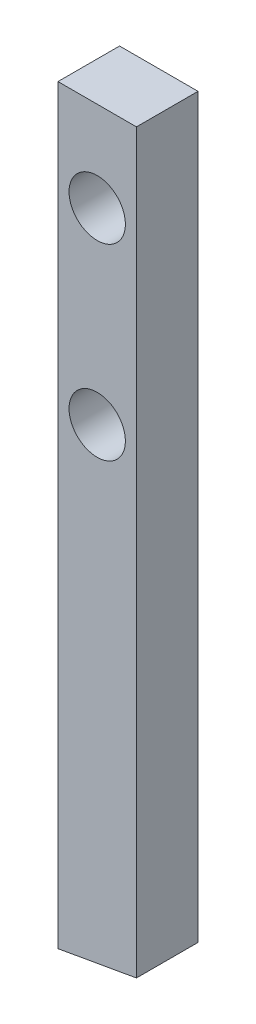
from build123d import *

# Parameters (mm, degrees)
SKETCH1_W           = 4.18
SKETCH1_H           = 3.28
BOSS_EXTRUDE1_DEPTH = 40
CUT_EXTRUDE1_DEPTH  = 40
SKETCH3_R           = 1.5
CUT_EXTRUDE2_DEPTH  = 40


with BuildPart() as part:
    # Sketch1 → Boss-Extrude1 (new body)
    with BuildSketch(Plane(origin=(0, 0, 0), x_dir=(1, 0, 0), z_dir=(0, 1, 0))):
        Rectangle(SKETCH1_W, SKETCH1_H)
    extrude(amount=BOSS_EXTRUDE1_DEPTH)

    # Sketch2 → Cut-Extrude1 (cut)
    with BuildSketch(Plane.XY.offset(1.64)):
        Polygon((-2.09, 0), (2.09, 0), (2.09, 0.737046779), align=None)
    extrude(amount=-CUT_EXTRUDE1_DEPTH, mode=Mode.SUBTRACT)

    # Sketch3 → Cut-Extrude2 (cut)
    with BuildSketch(Plane(origin=(0, 0, -1.64), x_dir=(-1, 0, 0), z_dir=(0, 0, -1))):
        with Locations((0, 35.211206118)):
            Circle(SKETCH3_R)
        with Locations((0, 25.211206118)):
            Circle(SKETCH3_R)
    extrude(amount=-CUT_EXTRUDE2_DEPTH, mode=Mode.SUBTRACT)


solid = part.part
